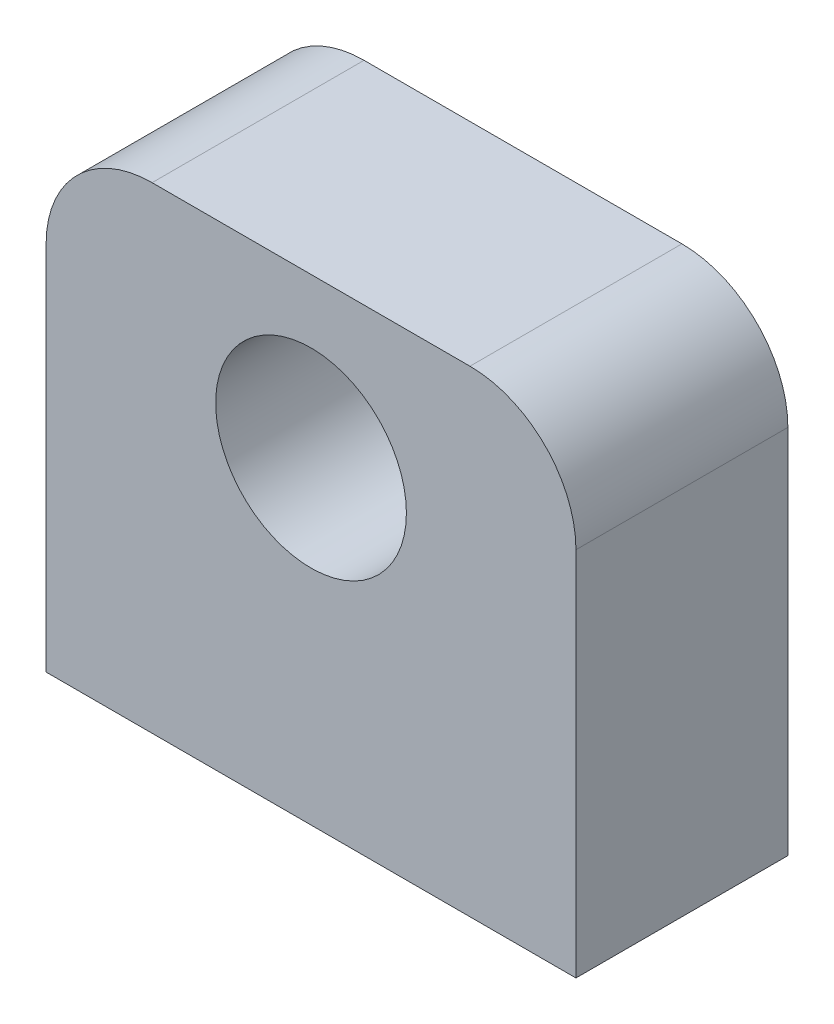
SolidWorks part; units mm, degrees
material "AISI 1010 钢，热轧条材"
ref_plane "Front Plane" through (0, 0, 0) normal (0, 0, 1) x (1, 0, 0)
ref_plane "Top Plane" through (0, 0, 0) normal (0, 1, 0) x (1, 0, 0)
ref_plane "Right Plane" through (0, 0, 0) normal (1, 0, 0) x (0, 0, -1)
sketch "Sketch1" plane through (0, 0, 0) normal (0, 0, 1) x (1, 0, 0)
  line L1 (0, 0) -> (50, 0)
  line L2 (0, 0) -> (0, 45)
  line L3 (0, 45) -> (50, 45)
  line L4 (50, 0) -> (50, 45)
  circle A0 centre (25, 30) radius 9
  dimension "D3" = 18
  dimension "D1" = 45
  dimension "D2" = 50
  dimension "D4" = 15
  dimension "D5" = 25
extrude "Boss-Extrude1" add sketch "Sketch1" along normal blind 20
fillet "Fillet1" radius 10 2 edges at (0, 45, 10) (50, 45, 10)
